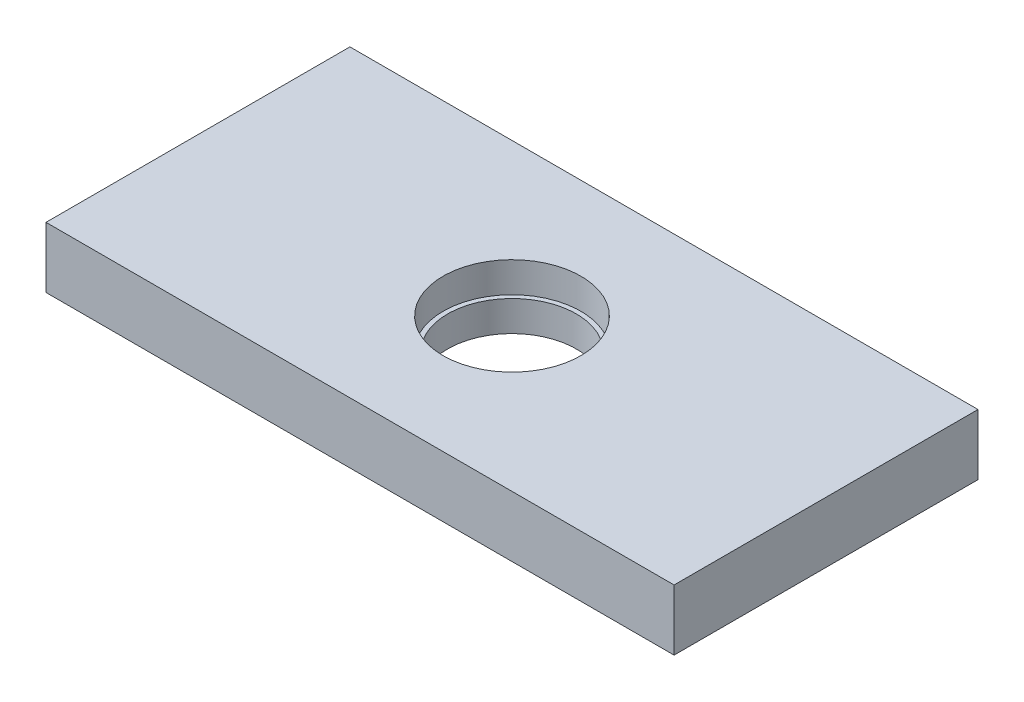
SolidWorks part; units mm, degrees
ref_plane "前视基准面" through (0, 0, 0) normal (0, 0, 1) x (1, 0, 0)
ref_plane "上视基准面" through (0, 0, 0) normal (0, 1, 0) x (1, 0, 0)
ref_plane "右视基准面" through (0, 0, 0) normal (1, 0, 0) x (0, 0, -1)
sketch "草图1" plane through (0, 0, 0) normal (0, 1, 0) x (1, 0, 0)
  line L1 (-155, -75) -> (155, -75)
  line L2 (-155, -75) -> (-155, 75)
  line L3 (-155, 75) -> (155, 75)
  line L4 (155, -75) -> (155, 75)
  line L5 (-155, -75) -> (155, 75) construction
  line L6 (-155, 75) -> (155, -75) construction
  point P0 (0, 0)
  dimension "D1" = 150
  dimension "D3" = 310
extrude "凸台-拉伸1" add sketch "草图1" along normal blind 30
sketch "草图2" plane through (0, 30, 0) normal (0, 1, 0) x (1, 0, 0)
  line L0 (155, -75) -> (155, 75) construction
  line L1 (155, 75) -> (-155, 75) construction
  circle A0 centre (0, 0) radius 31.75
  dimension "D1" = 63.5
  dimension "D2" = 155
  dimension "D3" = 75
extrude "切除-拉伸1" cut sketch "草图2" against normal through all
sketch "草图3" plane through (0, 30, 0) normal (0, 1, 0) x (1, 0, 0)
  line L0 (155, -75) -> (155, 75) construction
  line L1 (155, 75) -> (-155, 75) construction
  circle A0 centre (0, 0) radius 34
  dimension "D1" = 68
  dimension "D2" = 155
  dimension "D3" = 75
extrude "切除-拉伸2" cut sketch "草图3" against normal blind 15
